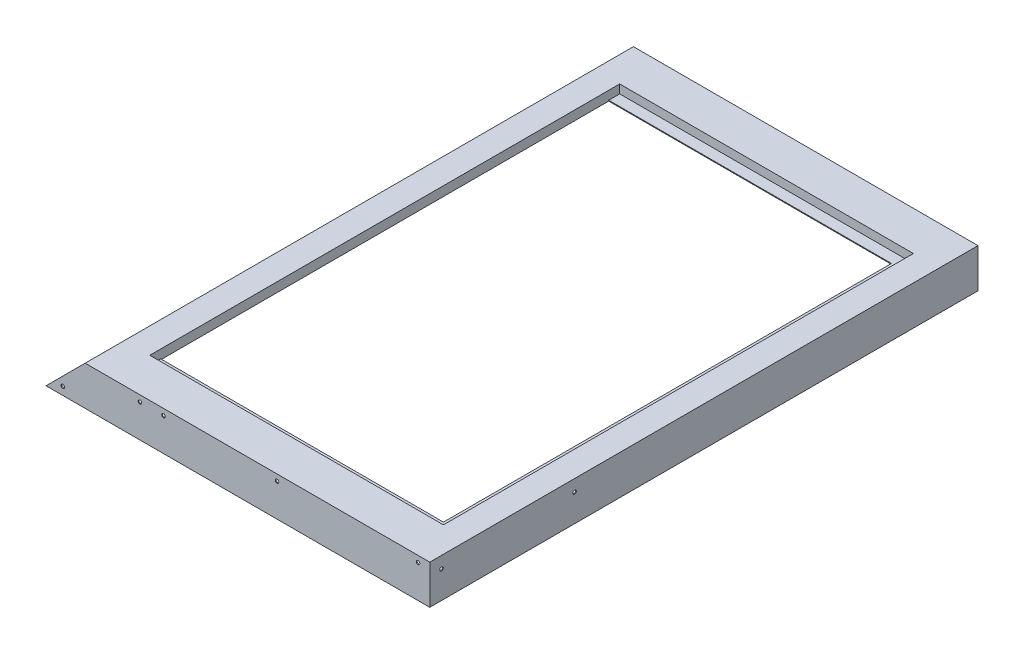
from build123d import *

# Parameters (mm, degrees)
EXTRUDE_1_DEPTH     = 700
SKETCH_2_W          = 750
SKETCH_2_H          = 1200
CUT_EXTRUDE_1_DEPTH = 43
SKETCH_3_W          = 754
SKETCH_3_H          = 1204
SKETCH_3_W_2        = 750
SKETCH_3_H_2        = 1200
EXTRUDE_2_DEPTH     = 24
EXTRUDE_3_DEPTH     = 2
EXTRUDE_4_DEPTH     = 2
SKETCH_6_W          = 980
SKETCH_6_H          = 30
EXTRUDE_5_DEPTH     = 2
EXTRUDE_7_DEPTH     = 2
SKETCH_9_R          = 4.5
CUT_EXTRUDE_2_DEPTH = 10
CUT_EXTRUDE_3_DEPTH = 45
SKETCH_11_R         = 4.5
CUT_EXTRUDE_4_DEPTH = 5
SKETCH_12_R         = 4.5
CUT_EXTRUDE_5_DEPTH = 10


with BuildPart() as part:
    # 草图1 → 凸台-拉伸1 (new, symmetric)
    with BuildSketch(Plane.XY):
        Polygon((490, 0), (460, 0), (460, 2), (488, 2), (488, 98), (-389.171572875, 98), (-485.171572875, 2), (-460, 2), (-460, 0), (-490, 0), (-390, 100), (490, 100), align=None)
    extrude(amount=EXTRUDE_1_DEPTH, both=True)

    # 草图2 → 切除-拉伸1 (cut)
    with BuildSketch(Plane(origin=(0, 100, 0), x_dir=(1, 0, 0), z_dir=(0, 1, 0))):
        with Locations((50, 0)):
            Rectangle(SKETCH_2_W, SKETCH_2_H)
    extrude(amount=-CUT_EXTRUDE_1_DEPTH, mode=Mode.SUBTRACT)

    # 草图3 → 凸台-拉伸2 (add)
    with BuildSketch(Plane(origin=(0, 100, 0), x_dir=(1, 0, 0), z_dir=(0, 1, 0))):
        with Locations((50, 0)):
            Rectangle(SKETCH_3_W, SKETCH_3_H)
        with Locations((50, 0)):
            Rectangle(SKETCH_3_W_2, SKETCH_3_H_2, mode=Mode.SUBTRACT)
    extrude(amount=-EXTRUDE_2_DEPTH)

    # 草图4 → 凸台-拉伸3 (add)
    with BuildSketch(Plane.XZ.offset(-76)):
        Polygon((-327, 602), (427, 602), (427, 572), (427, -572), (427, -602), (-327, -602), (-327, -572), (397, -572), (397, 0), (397, 572), (-327, 572), align=None)
    extrude(amount=-EXTRUDE_3_DEPTH)



with BuildPart() as body_2:
    # 草图5 → 凸台-拉伸4 (new body)
    with BuildSketch(Plane(origin=(0, 0, -700), x_dir=(-1, 0, 0), z_dir=(0, 0, -1))):
        Polygon((-490, 100), (-490, 0), (490, 0), (390, 100), align=None)
    extrude(amount=-EXTRUDE_4_DEPTH)


with BuildPart() as part_1:
    add(part.part)

    add(body_2.part)  # 凸台-拉伸5 merges body 2
    # 草图6 → 凸台-拉伸5 (add)
    with BuildSketch(Plane.XZ):
        with Locations((0, -685)):
            Rectangle(SKETCH_6_W, SKETCH_6_H)
    extrude(amount=-EXTRUDE_5_DEPTH)

    # 草图8 → 凸台-拉伸7 (add)
    with BuildSketch(Plane.XY.offset(700)):
        Polygon((490, 0), (490, 100), (-390, 100), (-490, 0), (-460, 0), (460, 0), align=None)
    extrude(amount=-EXTRUDE_7_DEPTH)

    # 草图9 → 切除-拉伸2 (cut)
    with BuildSketch(Plane(origin=(0, 0, 698), x_dir=(-1, 0, 0), z_dir=(0, 0, -1))):
        with Locations((-460, 84)):
            Circle(SKETCH_9_R)
        with Locations((250, 84)):
            Circle(SKETCH_9_R)
        with Locations((190, 84)):
            Circle(SKETCH_9_R)
        with Locations((447.012193309, 20.360389693)):
            Circle(SKETCH_9_R)
        with Locations((-100, 84)):
            Circle(SKETCH_9_R)
    extrude(amount=-CUT_EXTRUDE_2_DEPTH, mode=Mode.SUBTRACT)

    # 草图10 → 切除-拉伸3 (cut)
    with BuildSketch(Plane(origin=(0, 0, -700), x_dir=(-1, 0, 0), z_dir=(0, 0, -1))):
        Polygon((478.109799219, 11.890200781), (488, 2), (495.020614582, -5.020614582), (488.781283968, 5.695100391), align=None)
    extrude(amount=-CUT_EXTRUDE_3_DEPTH, mode=Mode.SUBTRACT)

    # 草图11 → 切除-拉伸4 (cut)
    with BuildSketch(Plane.XZ):
        with Locations((-474, 670)):
            Circle(SKETCH_11_R)
        with Locations((-474, 0)):
            Circle(SKETCH_11_R)
        with Locations((-474, -684)):
            Circle(SKETCH_11_R)
        with Locations((0, -684)):
            Circle(SKETCH_11_R)
        with Locations(Location((474, -684, 0), (0, 0, 270))):
            Circle(SKETCH_11_R)
        with Locations(Location((474, 0, 0), (0, 0, 270))):
            Circle(SKETCH_11_R)
        with Locations(Location((474, 670, 0), (0, 0, 270))):
            Circle(SKETCH_11_R)
    extrude(amount=-CUT_EXTRUDE_4_DEPTH, mode=Mode.SUBTRACT)

    # 草图12 → 切除-拉伸5 (cut)
    with BuildSketch(Plane.ZY.offset(-488)):
        with Locations((670, 70)):
            Circle(SKETCH_12_R)
        with Locations((330, 70)):
            Circle(SKETCH_12_R)
    extrude(amount=-CUT_EXTRUDE_5_DEPTH, mode=Mode.SUBTRACT)


solid = part_1.part
